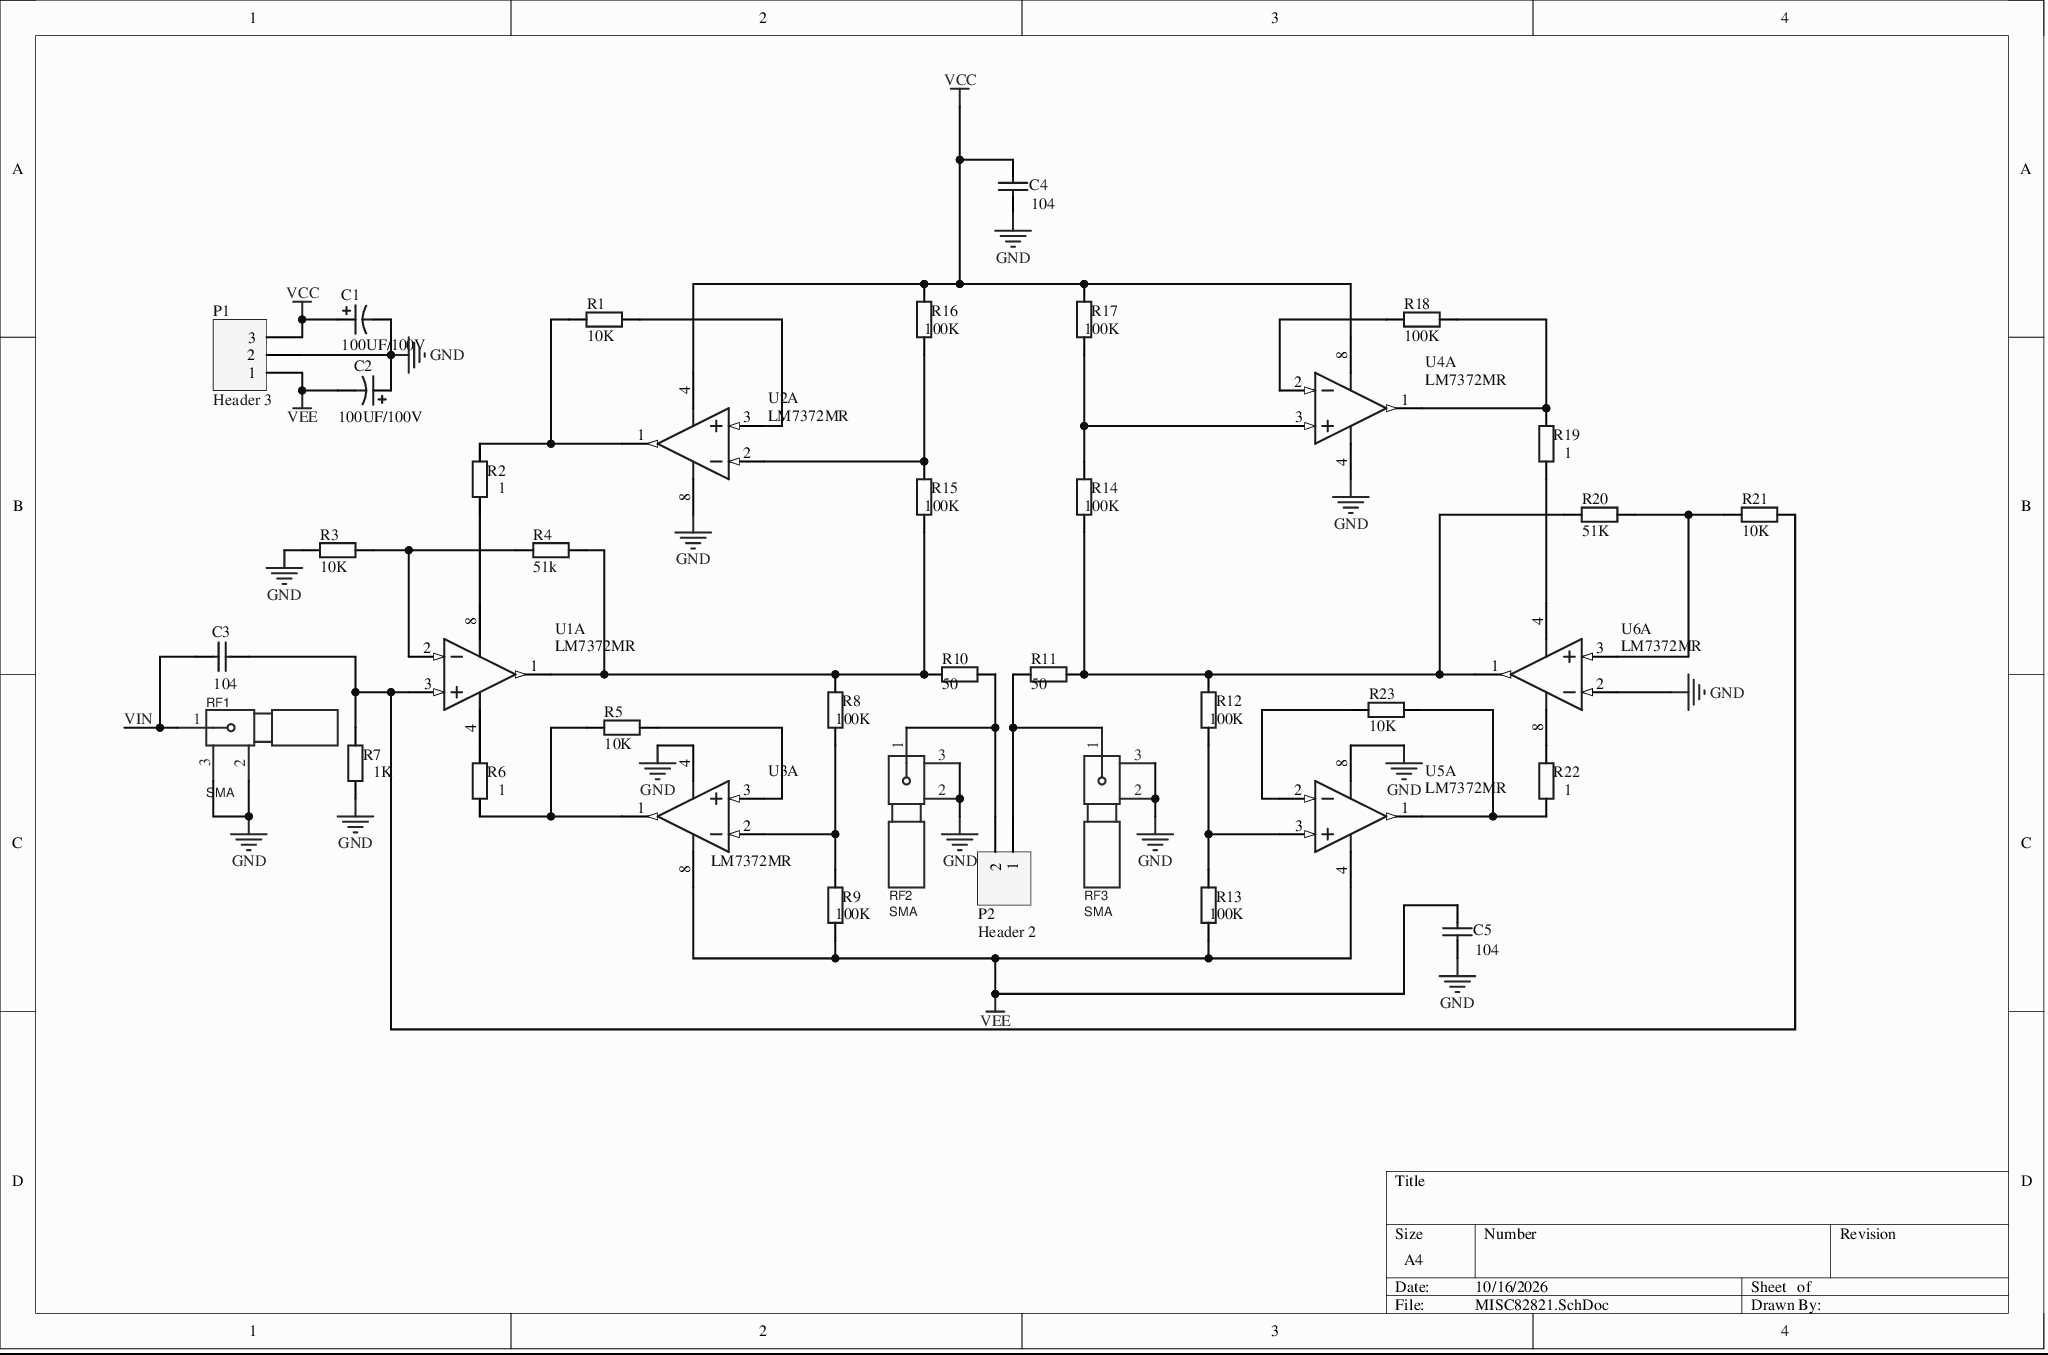
[diagram p0: MISC82821-10.SchDoc]
# Altium schematic sheet MISC82821-10.SchDoc
size A4

## Parts
C1  100UF/100V  [C0805]
C2  100UF/100V  [C0805]
C3  104  [C1206]
C4  104  [C1206]
C5  104  [C1206]
P1  Header 3  [HDR1X3]
P2  Header 2  [HDR1X2]
R1  10K  [AXIAL-0.4]
R2  1  [AXIAL-0.4]
R3  10K  [AXIAL-0.4]
R4  51k  [AXIAL-0.4]
R5  10K  [AXIAL-0.4]
R6  1  [AXIAL-0.4]
R7  1K  [AXIAL-0.4]
R8  100K  [AXIAL-0.4]
R9  100K  [AXIAL-0.4]
R10  50  [AXIAL-0.4]
R11  50  [AXIAL-0.4]
R12  100K  [AXIAL-0.4]
R13  100K  [AXIAL-0.4]
R14  100K  [AXIAL-0.4]
R15  100K  [AXIAL-0.4]
R16  100K  [AXIAL-0.4]
R17  100K  [AXIAL-0.4]
R18  100K  [AXIAL-0.4]
R19  1  [AXIAL-0.4]
R20  51K  [AXIAL-0.4]
R21  10K  [AXIAL-0.4]
R22  1  [AXIAL-0.4]
R23  10K  [AXIAL-0.4]
RF1  SMA  [SMA-SMD_HJ-SMA313]
RF2  SMA  [SMA-SMD_HJ-SMA313]
RF3  SMA  [SMA-SMD_HJ-SMA313]
U1  LM7372MR  [MRA08B_N]  (part A of 3)
U2  LM7372MR  [MRA08B_N]  (part A of 3)
U3  LM7372MR  [MRA08B_N]  (part A of 3)
U4  LM7372MR  [MRA08B_N]  (part A of 3)
U5  LM7372MR  [MRA08B_N]  (part A of 3)
U6  LM7372MR  [MRA08B_N]  (part A of 3)

## Nets
GND: C1.2 C2.1 C4.1 C5.1 P1.2 R3.1 R7.1 RF1.2 RF1.3 RF2.2 RF2.3 RF3.2 RF3.3 U2.8(V+) U3.4(V-) U4.4(V-) U5.8(V+) U6.2(INA-)
VCC: C1.1 C4.2 P1.3 R16.2 R17.2 U2.4(V-) U4.8(V+)
VEE: C2.2 C5.2 P1.1 R9.1 R13.1 U3.8(V+) U5.4(V-)
VIN: C3.2 RF1.1
NetC3_1: C3.1 R7.2 R21.2 U1.3(INA+)
NetP2_1: P2.1 R11.2 RF3.1
NetP2_2: P2.2 R10.1 RF2.1
NetR1_1: R1.1 R2.2 U2.1(OUTA)
NetR1_2: R1.2 U2.3(INA+)
NetR2_1: R2.1 U1.8(V+)
NetR3_2: R3.2 R4.1 U1.2(INA-)
NetR4_2: R4.2 R8.2 R10.2 R15.1 U1.1(OUTA)
NetR5_1: R5.1 R6.1 U3.1(OUTA)
NetR5_2: R5.2 U3.3(INA+)
NetR6_2: R6.2 U1.4(V-)
NetR8_1: R8.1 R9.2 U3.2(INA-)
NetR11_1: R11.1 R12.2 R14.1 R20.1 U6.1(OUTA)
NetR12_1: R12.1 R13.2 U5.3(INA+)
NetR14_2: R14.2 R17.1 U4.3(INA+)
NetR15_2: R15.2 R16.1 U2.2(INA-)
NetR18_1: R18.1 U4.2(INA-)
NetR18_2: R18.2 R19.2 U4.1(OUTA)
NetR19_1: R19.1 U6.4(V-)
NetR20_2: R20.2 R21.1 U6.3(INA+)
NetR22_1: R22.1 R23.2 U5.1(OUTA)
NetR22_2: R22.2 U6.8(V+)
NetR23_1: R23.1 U5.2(INA-)

## Library data of the parts
C1 C2 = Cap Pol3: Polarized Capacitor (Surface Mount); Published: 8-Jun-2000; LatestRevisionDate: 29-May-2009; LatestRevisionNote: IPC-7351 Footprint Added.; PackageReference: C0805; PackageDescription: Chip Capacitor; Value: 100UF/100V; Publisher: Altium Limited
C3-C5 = Cap Semi: Capacitor (Semiconductor SIM Model); Published: 8-Jun-2000; LatestRevisionDate: 29-May-2009; LatestRevisionNote: IPC-7351 Footprint Added.; PackageReference: C1206; PackageDescription: Chip Capacitor; Value: 104; Publisher: Altium Limited
P1 = Header 3: Header, 3-Pin; LatestRevisionDate: 17-Jul-2002; LatestRevisionNote: Re-released for DXP Platform.; Publisher: Altium Limited
P2 = Header 2: Header, 2-Pin; LatestRevisionDate: 17-Jul-2002; LatestRevisionNote: Re-released for DXP Platform.; Publisher: Altium Limited
R1-R17 R19-R23 = Res2: Resistor; Published: 8-Jun-2000; LatestRevisionDate: 17-Jul-2002; LatestRevisionNote: Re-released for DXP Platform.; PackageReference: AXIAL-0.4; PackageDescription: Axial Device, Thru-Hole; 2 Leads; 0.4 in Pin Spacing; Publisher: Altium Limited
  R1 R3 R5 R21 R23: Value: 10K
  R2 R6 R19 R22: Value: 1
  R4 R20: Value: 51K
  R7: Value: 1K
  R8 R9 R12-R17: Value: 100K
  R10 R11: Value: 50
R18 = Res2: Resistor; Value: 10K; Published: 8-Jun-2000; LatestRevisionDate: 17-Jul-2002; LatestRevisionNote: Re-released for DXP Platform.; PackageReference: AXIAL-0.4; PackageDescription: Axial Device, Thru-Hole; 2 Leads; 0.4 in Pin Spacing; Publisher: Altium Limited
RF1 RF3 = SMB: Antenna
RF2 = SMB: TI antenna
U1-U6 = LM7372MR: High Speed, High Output Current, Dual Operational Amplifier, 9-pin PSOP; Manufacturer: National Semiconductor; PackageTopMarking: NSXYTT*LM73*72MR; PowerWise: N; CompType: Amplifiers; Published: 4-Dec-2008; LatestRevisionDate: 13-Jan-2009; LatestRevisionNote: Sim Model Added.; DatasheetVersion: Jun-2008; PackageVersion: revB, Dec-2007; PackageReference: MRA08B; PackageDescription: Molded, PSOP .193 x .154 x .058in, 8 Lead, .050in Pitch, Large DAP; PartNumber: LM7372MR; RoHS: N; PinCount: 8; Code_JEDEC: MS-012-AA; ComponentLink1Description: LM7372 Datasheet; ComponentLink1URL: http://www.national.com/ds/LM/LM7372.pdf; ComponentLink2Description: LM7372 Web Page; ComponentLink2URL: http://www.national.com/pf/LM/LM7372.html; ComponentLink3Description: MRA08B Package Page; ComponentLink3URL: http://www.national.com/packaging/folders/mra08b.html; Publisher: Altium Limited